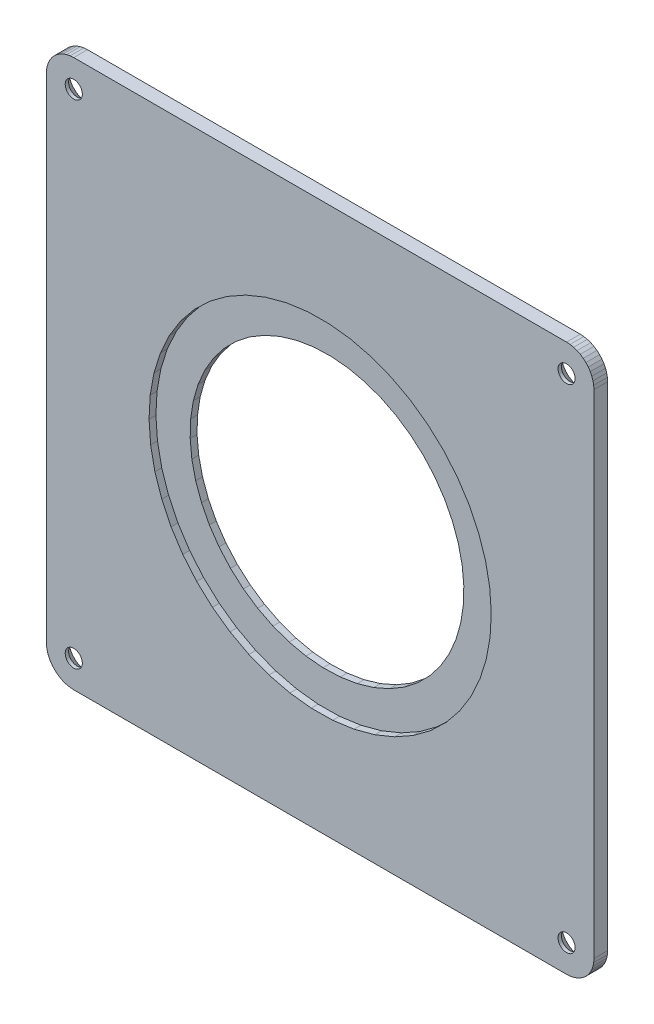
SolidWorks part; units mm, degrees
ref_plane "Front Plane" through (0, 0, 0) normal (0, 0, 1) x (1, 0, 0)
ref_plane "Top Plane" through (0, 0, 0) normal (0, 1, 0) x (1, 0, 0)
ref_plane "Right Plane" through (0, 0, 0) normal (1, 0, 0) x (0, 0, -1)
ref_plane "Plane1" through (0, 0, 37.0806) normal (0, 0, 1) x (1, 0, 0)
sketch "Sketch1" plane through (0, 0, 37.0806) normal (0, 0, 1) x (1, 0, 0)
  line L0 (-40, -36) -> (-39.9658, -36.5221)
  line L1 (-39.9658, -36.5221) -> (-39.8637, -37.0353)
  line L2 (-39.8637, -37.0353) -> (-39.6955, -37.5307)
  line L3 (-39.6955, -37.5307) -> (-39.4641, -38)
  line L4 (-39.4641, -38) -> (-39.1734, -38.435)
  line L5 (-39.1734, -38.435) -> (-38.8284, -38.8284)
  line L6 (-38.8284, -38.8284) -> (-38.435, -39.1734)
  line L7 (-38.435, -39.1734) -> (-38, -39.4641)
  line L8 (-38, -39.4641) -> (-37.5307, -39.6955)
  line L9 (-37.5307, -39.6955) -> (-37.0353, -39.8637)
  line L10 (-37.0353, -39.8637) -> (-36.5221, -39.9658)
  line L11 (-36.5221, -39.9658) -> (-36, -40)
  line L12 (-36, -40) -> (36, -40)
  line L13 (36, -40) -> (36.5221, -39.9658)
  line L14 (36.5221, -39.9658) -> (37.0353, -39.8637)
  line L15 (37.0353, -39.8637) -> (37.5307, -39.6955)
  line L16 (37.5307, -39.6955) -> (38, -39.4641)
  line L17 (38, -39.4641) -> (38.435, -39.1734)
  line L18 (38.435, -39.1734) -> (38.8284, -38.8284)
  line L19 (38.8284, -38.8284) -> (39.1734, -38.435)
  line L20 (39.1734, -38.435) -> (39.4641, -38)
  line L21 (39.4641, -38) -> (39.6955, -37.5307)
  line L22 (39.6955, -37.5307) -> (39.8637, -37.0353)
  line L23 (39.8637, -37.0353) -> (39.9658, -36.5221)
  line L24 (39.9658, -36.5221) -> (40, -36)
  line L25 (40, -36) -> (40, 36)
  line L26 (40, 36) -> (39.9658, 36.5221)
  line L27 (39.9658, 36.5221) -> (39.8637, 37.0353)
  line L28 (39.8637, 37.0353) -> (39.6955, 37.5307)
  line L29 (39.6955, 37.5307) -> (39.4641, 38)
  line L30 (39.4641, 38) -> (39.1734, 38.435)
  line L31 (39.1734, 38.435) -> (38.8284, 38.8284)
  line L32 (38.8284, 38.8284) -> (38.435, 39.1734)
  line L33 (38.435, 39.1734) -> (38, 39.4641)
  line L34 (38, 39.4641) -> (37.5307, 39.6955)
  line L35 (37.5307, 39.6955) -> (37.0353, 39.8637)
  line L36 (37.0353, 39.8637) -> (36.5221, 39.9658)
  line L37 (36.5221, 39.9658) -> (36, 40)
  line L38 (36, 40) -> (-36, 40)
  line L39 (-36, 40) -> (-36.5221, 39.9658)
  line L40 (-36.5221, 39.9658) -> (-37.0353, 39.8637)
  line L41 (-37.0353, 39.8637) -> (-37.5307, 39.6955)
  line L42 (-37.5307, 39.6955) -> (-38, 39.4641)
  line L43 (-38, 39.4641) -> (-38.435, 39.1734)
  line L44 (-38.435, 39.1734) -> (-38.8284, 38.8284)
  line L45 (-38.8284, 38.8284) -> (-39.1734, 38.435)
  line L46 (-39.1734, 38.435) -> (-39.4641, 38)
  line L47 (-39.4641, 38) -> (-39.6955, 37.5307)
  line L48 (-39.6955, 37.5307) -> (-39.8637, 37.0353)
  line L49 (-39.8637, 37.0353) -> (-39.9658, 36.5221)
  line L50 (-39.9658, 36.5221) -> (-40, 36)
  line L51 (-40, 36) -> (-40, -36)
extrude "Boss-Extrude1" add sketch "Sketch1" against normal blind 2
sketch "Sketch2" plane through (0, 0, 37.0806) normal (0, 0, 1) x (1, 0, 0)
  line L0 (-37.4489, -36.3882) -> (-37.299, -36.75)
  line L1 (-37.299, -36.75) -> (-37.0607, -37.0607)
  line L2 (-37.0607, -37.0607) -> (-36.75, -37.299)
  line L3 (-36.75, -37.299) -> (-36.3882, -37.4489)
  line L4 (-36.3882, -37.4489) -> (-36, -37.5)
  line L5 (-36, -37.5) -> (-35.6118, -37.4489)
  line L6 (-35.6118, -37.4489) -> (-35.25, -37.299)
  line L7 (-35.25, -37.299) -> (-34.9393, -37.0607)
  line L8 (-34.9393, -37.0607) -> (-34.701, -36.75)
  line L9 (-34.701, -36.75) -> (-34.5511, -36.3882)
  line L10 (-34.5511, -36.3882) -> (-34.5, -36)
  line L11 (-34.5, -36) -> (-34.5511, -35.6118)
  line L12 (-34.5511, -35.6118) -> (-34.701, -35.25)
  line L13 (-34.701, -35.25) -> (-34.9393, -34.9393)
  line L14 (-34.9393, -34.9393) -> (-35.25, -34.701)
  line L15 (-35.25, -34.701) -> (-35.6118, -34.5511)
  line L16 (-35.6118, -34.5511) -> (-36, -34.5)
  line L17 (-36, -34.5) -> (-36.3882, -34.5511)
  line L18 (-36.3882, -34.5511) -> (-36.75, -34.701)
  line L19 (-36.75, -34.701) -> (-37.0607, -34.9393)
  line L20 (-37.0607, -34.9393) -> (-37.299, -35.25)
  line L21 (-37.299, -35.25) -> (-37.4489, -35.6118)
  line L22 (-37.4489, -35.6118) -> (-37.5, -36)
  line L23 (-37.5, -36) -> (-37.4489, -36.3882)
extrude "Cut-Extrude1" cut sketch "Sketch2" against normal through all
sketch "Sketch3" plane through (0, 0, 37.0806) normal (0, 0, 1) x (1, 0, 0)
  line L0 (-37.4489, 35.6118) -> (-37.299, 35.25)
  line L1 (-37.299, 35.25) -> (-37.0607, 34.9393)
  line L2 (-37.0607, 34.9393) -> (-36.75, 34.701)
  line L3 (-36.75, 34.701) -> (-36.3882, 34.5511)
  line L4 (-36.3882, 34.5511) -> (-36, 34.5)
  line L5 (-36, 34.5) -> (-35.6118, 34.5511)
  line L6 (-35.6118, 34.5511) -> (-35.25, 34.701)
  line L7 (-35.25, 34.701) -> (-34.9393, 34.9393)
  line L8 (-34.9393, 34.9393) -> (-34.701, 35.25)
  line L9 (-34.701, 35.25) -> (-34.5511, 35.6118)
  line L10 (-34.5511, 35.6118) -> (-34.5, 36)
  line L11 (-34.5, 36) -> (-34.5511, 36.3882)
  line L12 (-34.5511, 36.3882) -> (-34.701, 36.75)
  line L13 (-34.701, 36.75) -> (-34.9393, 37.0607)
  line L14 (-34.9393, 37.0607) -> (-35.25, 37.299)
  line L15 (-35.25, 37.299) -> (-35.6118, 37.4489)
  line L16 (-35.6118, 37.4489) -> (-36, 37.5)
  line L17 (-36, 37.5) -> (-36.3882, 37.4489)
  line L18 (-36.3882, 37.4489) -> (-36.75, 37.299)
  line L19 (-36.75, 37.299) -> (-37.0607, 37.0607)
  line L20 (-37.0607, 37.0607) -> (-37.299, 36.75)
  line L21 (-37.299, 36.75) -> (-37.4489, 36.3882)
  line L22 (-37.4489, 36.3882) -> (-37.5, 36)
  line L23 (-37.5, 36) -> (-37.4489, 35.6118)
extrude "Cut-Extrude2" cut sketch "Sketch3" against normal through all
sketch "Sketch4" plane through (0, 0, 37.0806) normal (0, 0, 1) x (1, 0, 0)
  line L0 (34.7878, -36.8835) -> (35.0578, -37.1671)
  line L1 (35.0578, -37.1671) -> (35.392, -37.3712)
  line L2 (35.392, -37.3712) -> (35.7676, -37.4819)
  line L3 (35.7676, -37.4819) -> (36, -37.4876)
  line L4 (36, -37.4876) -> (36.1591, -37.4915)
  line L5 (36.1591, -37.4915) -> (36.5397, -37.3996)
  line L6 (36.5397, -37.3996) -> (36.8835, -37.2122)
  line L7 (36.8835, -37.2122) -> (37.1672, -36.9422)
  line L8 (37.1672, -36.9422) -> (37.3713, -36.6081)
  line L9 (37.3713, -36.6081) -> (37.4819, -36.2324)
  line L10 (37.4819, -36.2324) -> (37.4916, -35.841)
  line L11 (37.4916, -35.841) -> (37.3996, -35.4603)
  line L12 (37.3996, -35.4603) -> (37.2122, -35.1165)
  line L13 (37.2122, -35.1165) -> (36.9422, -34.8329)
  line L14 (36.9422, -34.8329) -> (36.608, -34.6288)
  line L15 (36.608, -34.6288) -> (36.2324, -34.5181)
  line L16 (36.2324, -34.5181) -> (35.8409, -34.5085)
  line L17 (35.8409, -34.5085) -> (35.4603, -34.6004)
  line L18 (35.4603, -34.6004) -> (35.1165, -34.7878)
  line L19 (35.1165, -34.7878) -> (34.8329, -35.0578)
  line L20 (34.8329, -35.0578) -> (34.6288, -35.392)
  line L21 (34.6288, -35.392) -> (34.5181, -35.7676)
  line L22 (34.5181, -35.7676) -> (34.5085, -36.1591)
  line L23 (34.5085, -36.1591) -> (34.6004, -36.5397)
  line L24 (34.6004, -36.5397) -> (34.7878, -36.8835)
extrude "Cut-Extrude3" cut sketch "Sketch4" against normal through all
sketch "Sketch5" plane through (0, 0, 35.0806) normal (0, 0, -1) x (-1, 0, 0)
  line L0 (-36.3882, 37.4489) -> (-36.75, 37.299)
  line L1 (-36.75, 37.299) -> (-37.0607, 37.0607)
  line L2 (-37.0607, 37.0607) -> (-37.299, 36.75)
  line L3 (-37.299, 36.75) -> (-37.4489, 36.3882)
  line L4 (-37.4489, 36.3882) -> (-37.5, 36)
  line L5 (-37.5, 36) -> (-37.4489, 35.6118)
  line L6 (-37.4489, 35.6118) -> (-37.299, 35.25)
  line L7 (-37.299, 35.25) -> (-37.0607, 34.9393)
  line L8 (-37.0607, 34.9393) -> (-36.75, 34.701)
  line L9 (-36.75, 34.701) -> (-36.3882, 34.5511)
  line L10 (-36.3882, 34.5511) -> (-36, 34.5)
  line L11 (-36, 34.5) -> (-35.6118, 34.5511)
  line L12 (-35.6118, 34.5511) -> (-35.25, 34.701)
  line L13 (-35.25, 34.701) -> (-34.9393, 34.9393)
  line L14 (-34.9393, 34.9393) -> (-34.701, 35.25)
  line L15 (-34.701, 35.25) -> (-34.5511, 35.6118)
  line L16 (-34.5511, 35.6118) -> (-34.5, 36)
  line L17 (-34.5, 36) -> (-34.5511, 36.3882)
  line L18 (-34.5511, 36.3882) -> (-34.701, 36.75)
  line L19 (-34.701, 36.75) -> (-34.9393, 37.0607)
  line L20 (-34.9393, 37.0607) -> (-35.25, 37.299)
  line L21 (-35.25, 37.299) -> (-35.6118, 37.4489)
  line L22 (-35.6118, 37.4489) -> (-36, 37.5)
  line L23 (-36, 37.5) -> (-36.3882, 37.4489)
extrude "Cut-Extrude4" cut sketch "Sketch5" against normal through all
sketch "Sketch6" plane through (0, 0, 37.0806) normal (0, 0, 1) x (1, 0, 0)
  line L0 (-23.1462, -9.4474) -> (-21.7796, -12.2739)
  line L1 (-21.7796, -12.2739) -> (-20.0695, -14.9069)
  line L2 (-20.0695, -14.9069) -> (-18.0429, -17.3047)
  line L3 (-18.0429, -17.3047) -> (-15.7318, -19.4296)
  line L4 (-15.7318, -19.4296) -> (-13.1726, -21.2481)
  line L5 (-13.1726, -21.2481) -> (-10.4056, -22.7315)
  line L6 (-10.4056, -22.7315) -> (-7.4745, -23.8565)
  line L7 (-7.4745, -23.8565) -> (-4.4256, -24.6052)
  line L8 (-4.4256, -24.6052) -> (-1.3069, -24.9658)
  line L9 (-1.3069, -24.9658) -> (1.8325, -24.9327)
  line L10 (1.8325, -24.9327) -> (4.9429, -24.5065)
  line L11 (4.9429, -24.5065) -> (7.9754, -23.6937)
  line L12 (7.9754, -23.6937) -> (10.8822, -22.5073)
  line L13 (10.8822, -22.5073) -> (13.6173, -20.9659)
  line L14 (13.6173, -20.9659) -> (16.1376, -19.0939)
  line L15 (16.1376, -19.0939) -> (18.4035, -16.9208)
  line L16 (18.4035, -16.9208) -> (20.3791, -14.4808)
  line L17 (20.3791, -14.4808) -> (22.0333, -11.8124)
  line L18 (22.0333, -11.8124) -> (23.3401, -8.9578)
  line L19 (23.3401, -8.9578) -> (24.2787, -5.9618)
  line L20 (24.2787, -5.9618) -> (24.8345, -2.8719)
  line L21 (24.8345, -2.8719) -> (24.9986, 0.2633)
  line L22 (24.9986, 0.2633) -> (24.7685, 3.3944)
  line L23 (24.7685, 3.3944) -> (24.1477, 6.472)
  line L24 (24.1477, 6.472) -> (23.1462, 9.4474)
  line L25 (23.1462, 9.4474) -> (21.7796, 12.2739)
  line L26 (21.7796, 12.2739) -> (20.0695, 14.9069)
  line L27 (20.0695, 14.9069) -> (18.0429, 17.3047)
  line L28 (18.0429, 17.3047) -> (15.7318, 19.4296)
  line L29 (15.7318, 19.4296) -> (13.1726, 21.2481)
  line L30 (13.1726, 21.2481) -> (10.4056, 22.7315)
  line L31 (10.4056, 22.7315) -> (7.4745, 23.8565)
  line L32 (7.4745, 23.8565) -> (4.4256, 24.6052)
  line L33 (4.4256, 24.6052) -> (1.3069, 24.9658)
  line L34 (1.3069, 24.9658) -> (-1.8325, 24.9327)
  line L35 (-1.8325, 24.9327) -> (-4.9429, 24.5065)
  line L36 (-4.9429, 24.5065) -> (-7.9754, 23.6937)
  line L37 (-7.9754, 23.6937) -> (-10.8822, 22.5073)
  line L38 (-10.8822, 22.5073) -> (-13.6173, 20.9659)
  line L39 (-13.6173, 20.9659) -> (-16.1376, 19.0939)
  line L40 (-16.1376, 19.0939) -> (-18.4035, 16.9208)
  line L41 (-18.4035, 16.9208) -> (-20.3791, 14.4808)
  line L42 (-20.3791, 14.4808) -> (-22.0333, 11.8124)
  line L43 (-22.0333, 11.8124) -> (-23.3401, 8.9578)
  line L44 (-23.3401, 8.9578) -> (-24.2787, 5.9618)
  line L45 (-24.2787, 5.9618) -> (-24.8345, 2.8719)
  line L46 (-24.8345, 2.8719) -> (-24.9986, -0.2633)
  line L47 (-24.9986, -0.2633) -> (-24.7685, -3.3944)
  line L48 (-24.7685, -3.3944) -> (-24.1477, -6.472)
  line L49 (-24.1477, -6.472) -> (-23.1462, -9.4474)
extrude "Cut-Extrude5" cut sketch "Sketch6" against normal blind 1
sketch "Sketch7" plane through (0, 0, 36.0806) normal (0, 0, 1) x (1, 0, 0)
  line L0 (-19.7448, -3.1847) -> (-19.19, -5.6343)
  line L1 (-19.19, -5.6343) -> (-18.3325, -7.995)
  line L2 (-18.3325, -7.995) -> (-17.1859, -10.2296)
  line L3 (-17.1859, -10.2296) -> (-15.7683, -12.3029)
  line L4 (-15.7683, -12.3029) -> (-14.102, -14.1822)
  line L5 (-14.102, -14.1822) -> (-12.2133, -15.8378)
  line L6 (-12.2133, -15.8378) -> (-10.1319, -17.2437)
  line L7 (-10.1319, -17.2437) -> (-7.8908, -18.3776)
  line L8 (-7.8908, -18.3776) -> (-5.5253, -19.2216)
  line L9 (-5.5253, -19.2216) -> (-3.0726, -19.7626)
  line L10 (-3.0726, -19.7626) -> (-0.5715, -19.9918)
  line L11 (-0.5715, -19.9918) -> (1.9387, -19.9058)
  line L12 (1.9387, -19.9058) -> (4.4182, -19.5059)
  line L13 (4.4182, -19.5059) -> (6.8281, -18.7983)
  line L14 (6.8281, -18.7983) -> (9.1303, -17.7943)
  line L15 (9.1303, -17.7943) -> (11.2886, -16.5096)
  line L16 (11.2886, -16.5096) -> (13.2688, -14.9646)
  line L17 (13.2688, -14.9646) -> (15.0397, -13.1836)
  line L18 (15.0397, -13.1836) -> (16.5734, -11.1947)
  line L19 (16.5734, -11.1947) -> (17.8458, -9.0292)
  line L20 (17.8458, -9.0292) -> (18.8368, -6.7213)
  line L21 (18.8368, -6.7213) -> (19.5306, -4.3075)
  line L22 (19.5306, -4.3075) -> (19.9165, -1.8257)
  line L23 (19.9165, -1.8257) -> (19.9883, 0.6849)
  line L24 (19.9883, 0.6849) -> (19.7448, 3.1847)
  line L25 (19.7448, 3.1847) -> (19.19, 5.6343)
  line L26 (19.19, 5.6343) -> (18.3325, 7.995)
  line L27 (18.3325, 7.995) -> (17.1859, 10.2296)
  line L28 (17.1859, 10.2296) -> (15.7683, 12.3029)
  line L29 (15.7683, 12.3029) -> (14.102, 14.1822)
  line L30 (14.102, 14.1822) -> (12.2133, 15.8378)
  line L31 (12.2133, 15.8378) -> (10.1319, 17.2437)
  line L32 (10.1319, 17.2437) -> (7.8908, 18.3776)
  line L33 (7.8908, 18.3776) -> (5.5253, 19.2216)
  line L34 (5.5253, 19.2216) -> (3.0726, 19.7626)
  line L35 (3.0726, 19.7626) -> (0.5715, 19.9918)
  line L36 (0.5715, 19.9918) -> (-1.9387, 19.9058)
  line L37 (-1.9387, 19.9058) -> (-4.4182, 19.5059)
  line L38 (-4.4182, 19.5059) -> (-6.8281, 18.7983)
  line L39 (-6.8281, 18.7983) -> (-9.1303, 17.7943)
  line L40 (-9.1303, 17.7943) -> (-11.2886, 16.5096)
  line L41 (-11.2886, 16.5096) -> (-13.2688, 14.9646)
  line L42 (-13.2688, 14.9646) -> (-15.0397, 13.1836)
  line L43 (-15.0397, 13.1836) -> (-16.5734, 11.1947)
  line L44 (-16.5734, 11.1947) -> (-17.8458, 9.0292)
  line L45 (-17.8458, 9.0292) -> (-18.8368, 6.7213)
  line L46 (-18.8368, 6.7213) -> (-19.5306, 4.3075)
  line L47 (-19.5306, 4.3075) -> (-19.9165, 1.8257)
  line L48 (-19.9165, 1.8257) -> (-19.9883, -0.6849)
  line L49 (-19.9883, -0.6849) -> (-19.7448, -3.1847)
extrude "Cut-Extrude6" cut sketch "Sketch7" against normal through all
sketch "Sketch9" plane through (0, 0, 35.0806) normal (0, 0, -1) x (-1, 0, 0)
  line L0 (0, 0) -> (0, 40) construction
  line L1 (-36, 40) -> (36, 40) construction
  line L2 (0, 40) -> (0, 0) construction
  line L3 (0, 0) -> (40, 0) construction
  line L4 (40, 36) -> (40, -36) construction
  circle A0 centre (36, 36) radius 2
  circle A1 centre (36, -36) radius 2
  circle A2 centre (-36, -36) radius 2
  circle A3 centre (-36, 36) radius 2
  dimension "D1" = 4
  dimension "D2" = 72
extrude "Cut-Extrude7" cut sketch "Sketch9" against normal blind 10
other "Move Face1" face at (38, 36, 37.0806) face at (38, -36, 37.0806) face at (-34, -36, 37.0806) face at (-34, 36, 37.0806) parameters "D1"=0.75
chamfer "Chamfer1" distance 1.5 angle 45 4 edges at (-34.75, 36, 35.0806) (-34.75, -36, 35.0806) (37.25, -36, 35.0806) (37.25, 36, 35.0806)
